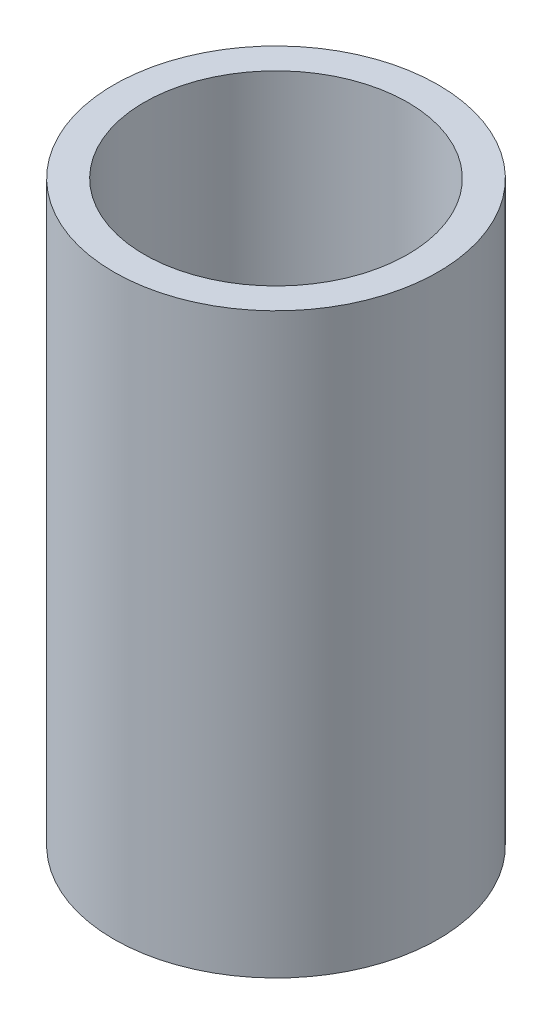
from build123d import *

# Parameters (mm, degrees)
SKETCH1_R           = 16
SKETCH1_R_2         = 13
BOSS_EXTRUDE1_DEPTH = 57


with BuildPart() as part:
    # Sketch1 → Boss-Extrude1 (new body)
    with BuildSketch(Plane(origin=(0, 0, 0), x_dir=(1, 0, 0), z_dir=(0, 1, 0))):
        with Locations(Location((0, 0, 0), (0, 0, 90))):
            Circle(SKETCH1_R)
        with Locations(Location((0, 0, 0), (0, 0, 90))):
            Circle(SKETCH1_R_2, mode=Mode.SUBTRACT)
    extrude(amount=BOSS_EXTRUDE1_DEPTH)


solid = part.part
